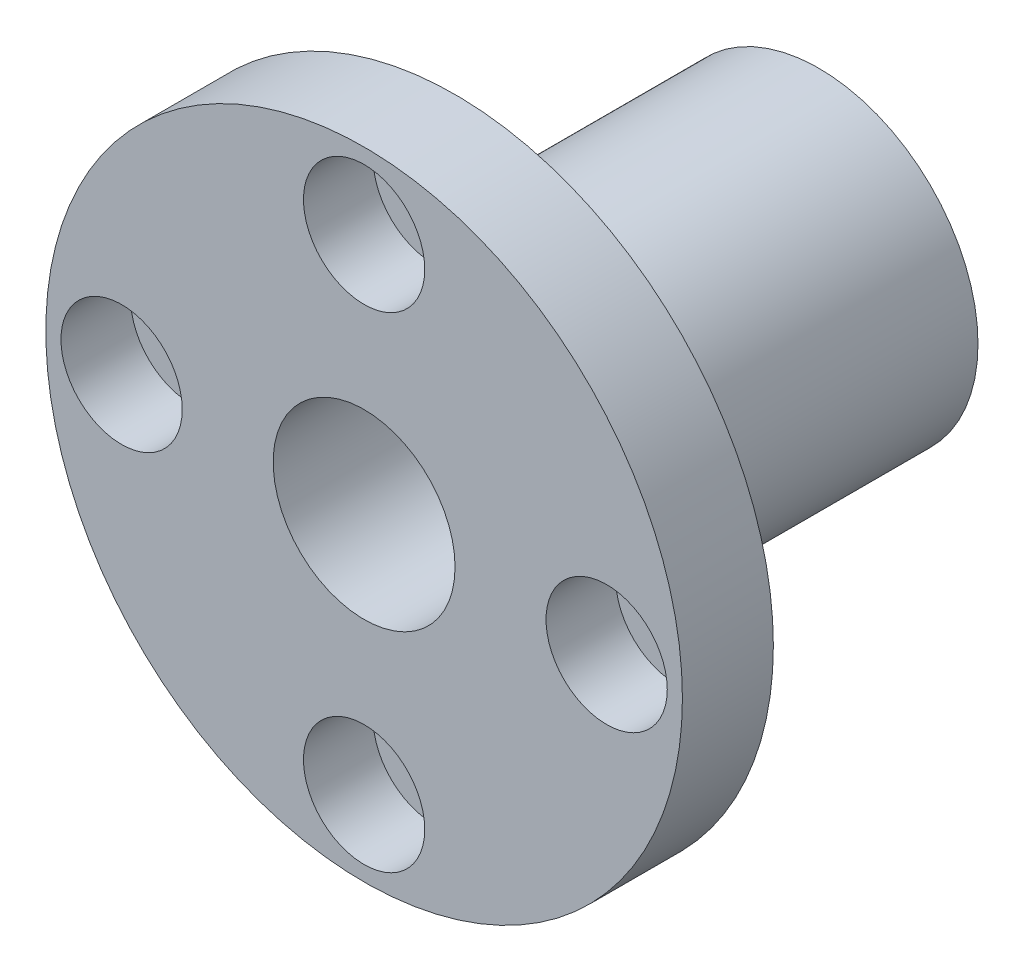
SolidWorks part; units mm, degrees
ref_plane "前视基准面" through (0, 0, 0) normal (0, 0, 1) x (1, 0, 0)
ref_plane "上视基准面" through (0, 0, 0) normal (0, 1, 0) x (1, 0, 0)
ref_plane "右视基准面" through (0, 0, 0) normal (1, 0, 0) x (0, 0, -1)
sketch "草图1" plane through (0, 0, 0) normal (0, 0, 1) x (1, 0, 0)
  circle A0 centre (0, 0) radius 10.5
  circle A1 centre (0, 0) radius 6
  dimension "D1" = 21
  dimension "D2" = 12
extrude "凸台-拉伸1" add sketch "草图1" along normal mid plane 30
sketch "草图2" plane through (0, 0, 15) normal (0, 0, 1) x (1, 0, 0)
  circle A0 centre (0, 0) radius 21
  circle A1 centre (0, 0) radius 10.5
  dimension "D1" = 42
  dimension "D2" = 21
extrude "凸台-拉伸2" add sketch "草图2" against normal blind 6
hole_wizard "打孔尺寸(%根据)内六角圆柱头螺钉的类型1" positions "草图6" profile "草图5" counterbore size "M4" standard "GB"
sketch "草图6" plane through (0, 0, 15) normal (0, 0, 1) x (1, 0, 0)
  circle A0 centre (0, 0) radius 16
  point P0 (0, 16)
  point P2 (16, 0)
  point P4 (0, -16)
  point P6 (-16, 0)
  dimension "D1" = 32
sketch "草图5" plane through (0, 16, 15) normal (1, 0, 0) x (0, -1, 0)
  line L0 (0, 0) -> (0, 12.8519)
  line L1 (0, 12.8519) -> (2.25, 11.5)
  line L2 (2.25, 11.5) -> (2.25, 4.6)
  line L3 (2.25, 4.6) -> (4, 4.6)
  line L4 (4, 4.6) -> (4, 0)
  line L5 (4, 0) -> (0, 0)
  line L10 (0, 12.8519) -> (-2.25, 11.5) construction
  line L11 (0, -6.35) -> (0, 107.95) construction
  dimension "孔直径" = 4.5
  dimension "孔深度" = 11.5
  dimension "柱形沉头孔直径" = 8
  dimension "柱形沉头孔深度" = 4.6
  dimension "导头角度" = 118
